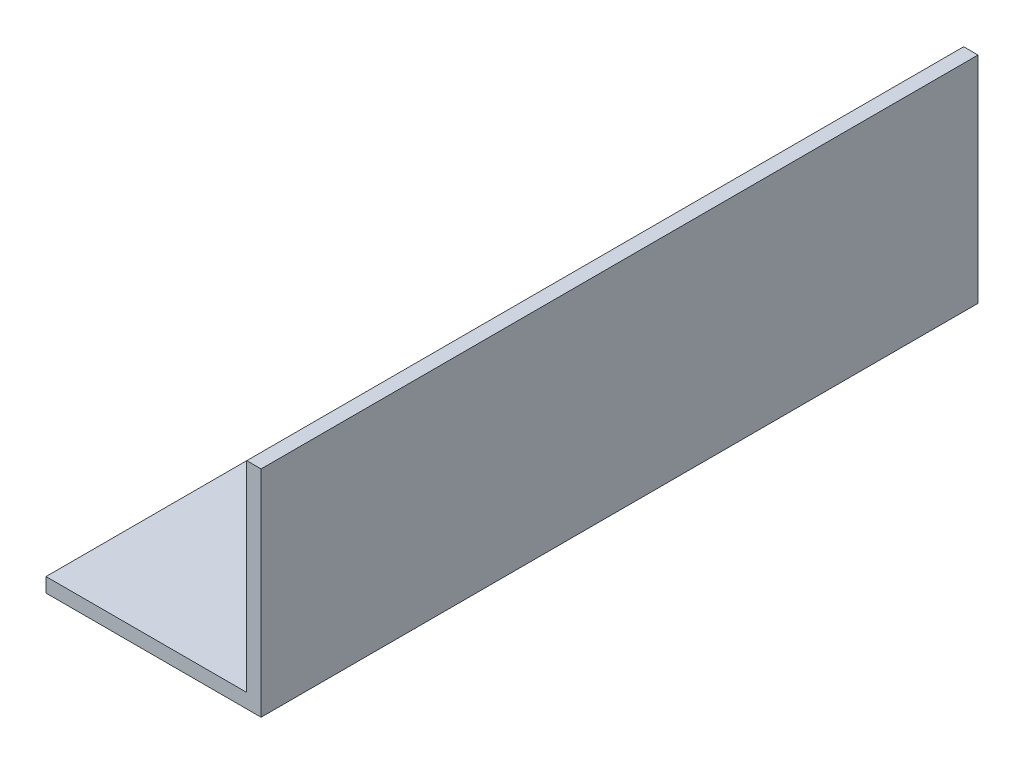
SolidWorks part; units mm, degrees
ref_plane "前视基准面" through (0, 0, 0) normal (0, 0, 1) x (1, 0, 0)
ref_plane "上视基准面" through (0, 0, 0) normal (0, 1, 0) x (1, 0, 0)
ref_plane "右视基准面" through (0, 0, 0) normal (1, 0, 0) x (0, 0, -1)
sketch "草图1" plane through (0, 0, 0) normal (0, 0, 1) x (1, 0, 0)
  line L0 (0, 0) -> (30, 0)
  line L1 (30, 0) -> (30, 30)
  line L2 (0, 2) -> (28, 2)
  line L3 (28, 2) -> (28, 30)
  line L4 (28, 30) -> (30, 30)
  line L5 (0, 0) -> (0, 2)
  dimension "D1" = 2
extrude "凸台-拉伸2" add sketch "草图1" along normal blind 100
